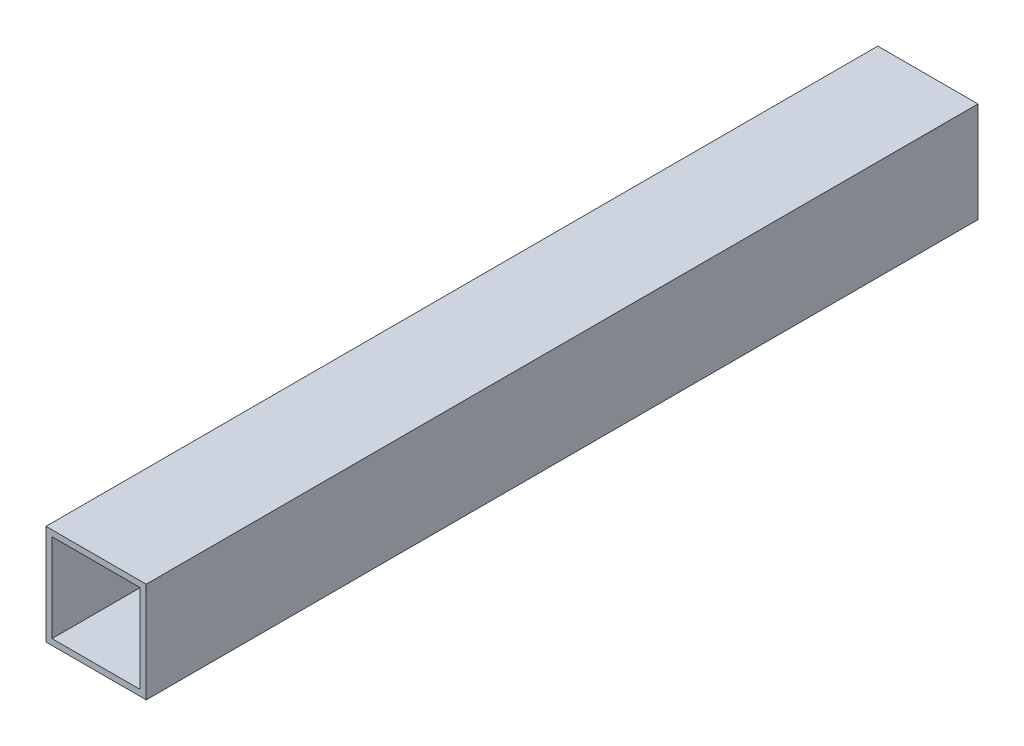
SolidWorks part; units mm, degrees
ref_plane "前视基准面" through (0, 0, 0) normal (0, 0, 1) x (1, 0, 0)
ref_plane "上视基准面" through (0, 0, 0) normal (0, 1, 0) x (1, 0, 0)
ref_plane "右视基准面" through (0, 0, 0) normal (1, 0, 0) x (0, 0, -1)
sketch "草图1" plane through (0, 0, 0) normal (0, 0, 1) x (1, 0, 0)
  line L0 (0, 0) -> (0, 50)
  line L1 (0, 50) -> (50, 50)
  line L2 (50, 50) -> (50, 0)
  line L3 (50, 0) -> (0, 0)
  line L4 (3, 3) -> (3, 47)
  line L5 (3, 47) -> (47, 47)
  line L6 (47, 47) -> (47, 3)
  line L7 (47, 3) -> (3, 3)
  dimension "D1" = 3
extrude "凸台-拉伸1" add sketch "草图1" along normal blind 415
